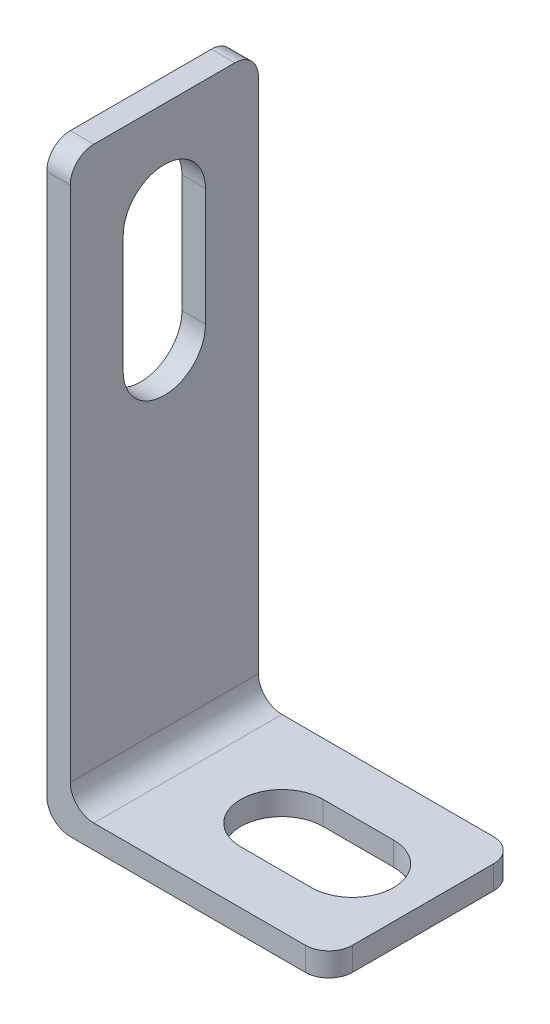
SolidWorks part; units mm, degrees
material "SUS304"
ref_plane "Front Plane" through (0, 0, 0) normal (0, 0, 1) x (1, 0, 0)
ref_plane "Top Plane" through (0, 0, 0) normal (0, 1, 0) x (1, 0, 0)
ref_plane "Right Plane" through (0, 0, 0) normal (1, 0, 0) x (0, 0, -1)
sketch "Sketch1" plane through (0, 0, 0) normal (0, 0, 1) x (1, 0, 0)
  line L0 (0, 0) -> (0, 25)
  line L1 (0, 0) -> (12, 0)
  dimension "D1" = 25
  dimension "D2" = 12
extrude "Extrude-Thin1" add sketch "Sketch1" along normal mid plane 8 thin
sketch "Sketch2" plane through (0, 1, 0) normal (0, 1, 0) x (1, 0, 0)
  line L0 (6, 0) -> (9, 0) construction
  line L1 (6, 1.75) -> (9, 1.75)
  line L2 (6, -1.75) -> (9, -1.75)
  line L3 (12, -4) -> (12, 4) construction
  arc A0 (6, 1.75) -> (6, -1.75) centre (6, 0) ccw
  arc A1 (9, -1.75) -> (9, 1.75) centre (9, 0) ccw
  point P3 (7.5, 0)
  dimension "D1" = 1.75
  dimension "D3" = 3
  dimension "D2" = 3
extrude "Cut-Extrude1" cut sketch "Sketch2" against normal through all
sketch "Sketch3" plane through (0, 0, 0) normal (-1, 0, 0) x (0, 0, 1)
  line L0 (0, 16) -> (0, 21) construction
  line L1 (-1.75, 16) -> (-1.75, 21)
  line L2 (1.75, 16) -> (1.75, 21)
  line L3 (4, 0) -> (-4, 0) construction
  arc A0 (-1.75, 16) -> (1.75, 16) centre (0, 16) ccw
  arc A1 (1.75, 21) -> (-1.75, 21) centre (0, 21) ccw
  point P3 (0, 18.5)
  dimension "D1" = 1.75
  dimension "D2" = 5
  dimension "D3" = 16
extrude "Cut-Extrude2" cut sketch "Sketch3" against normal through all
fillet "Fillet1" radius 1 6 edges at (0.5, 25, -4) (0.5, 25, 4) (12, 0.5, -4) (12, 0.5, 4) (0, 0, 0) (1, 1, 0)
